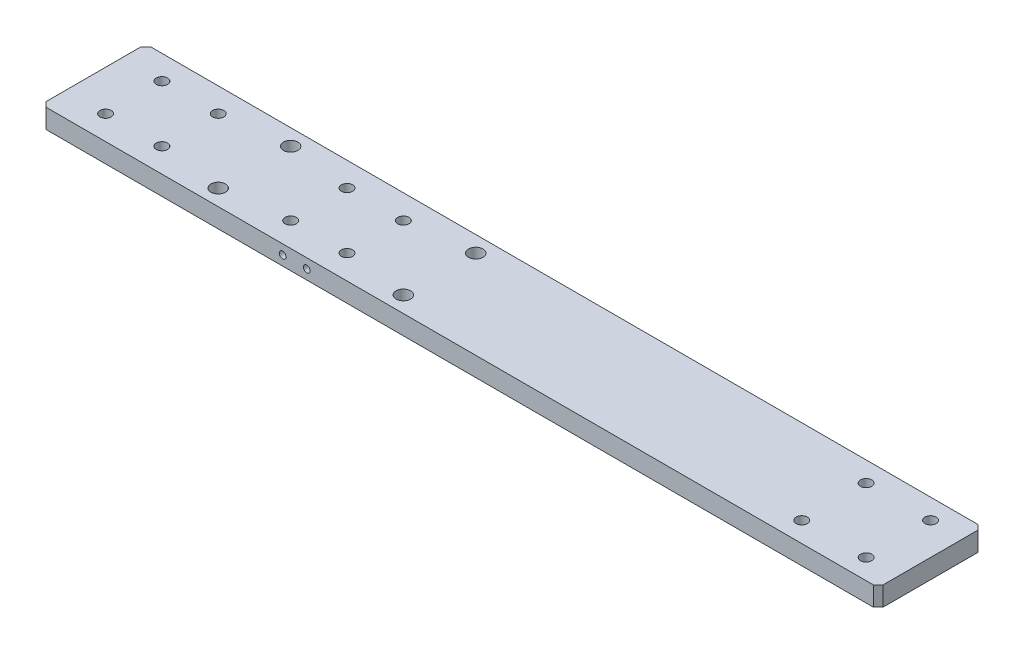
SolidWorks part; units mm, degrees
ref_plane "前视基准面" through (0, 0, 0) normal (0, 0, 1) x (1, 0, 0)
ref_plane "上视基准面" through (0, 0, 0) normal (0, 1, 0) x (1, 0, 0)
ref_plane "右视基准面" through (0, 0, 0) normal (1, 0, 0) x (0, 0, -1)
sketch "草图2" plane through (0, 0, 0) normal (0, 1, 0) x (1, 0, 0)
  line L1 (-260, 32.5) -> (260, 32.5)
  line L2 (-260, 32.5) -> (-260, -32.5)
  line L3 (-260, -32.5) -> (260, -32.5)
  line L4 (260, 32.5) -> (260, -32.5)
  line L5 (-260, 32.5) -> (260, -32.5) construction
  line L6 (-260, -32.5) -> (260, 32.5) construction
  point P0 (0, 0)
  dimension "D1" = 65
  dimension "D2" = 520
extrude "凸台-拉伸1" add sketch "草图2" along normal blind 12
hole_wizard "Ø7.0 (7) 直径孔1" positions "草图9" profile "草图8" hole size "Ø7.0" standard "GB" end condition through all
sketch "草图9" plane through (0, 0, 0) normal (0, 1, 0) x (1, 0, 0)
  line L0 (260, -32.5) -> (260, 32.5) construction
  point P0 (240, 20)
  point P2 (200, 20)
  point P4 (200, -20)
  point P6 (240, -20)
  dimension "D1" = 20
  dimension "D2" = 40
  dimension "D3" = 20
  dimension "D4" = 40
sketch "草图8" plane through (240, 0, -20) normal (1, 0, 0) x (0, 0, -1)
  line L0 (0, 0) -> (0, 12)
  line L1 (0, 12) -> (3.5, 12)
  line L2 (3.5, 12) -> (3.5, 0)
  line L5 (3.5, 0) -> (0, 0)
  line L11 (0, -6.35) -> (0, 107.95) construction
  dimension "通孔孔直径" = 7
  dimension "通孔孔深度" = 12
hole_wizard "M6 螺纹孔1" positions "草图11" profile "草图10" tap size "M6" standard "ISO"
sketch "草图11" plane through (-225, 0, 0) normal (-1, 0, 0) x (0, 0, 1)
  point P0 (0, 22)
  dimension "D1" = 22
cosmetic thread "孔螺蚊线1" [suppressed] parameters "D1"=17, "D2"=6
sketch "草图10" plane through (-225, 22, 0) normal (0, 1, 0) x (0, 0, 1)
  line L0 (0, 0) -> (0, 18.5022)
  line L1 (0, 18.5022) -> (2.5, 17)
  line L2 (2.5, 17) -> (2.5, 0)
  line L5 (2.5, 0) -> (0, 0)
  line L10 (0, 18.5022) -> (-2.5, 17) construction
  line L11 (0, -6.35) -> (0, 107.95) construction
  dimension "螺纹孔钻头直径" = 5
  dimension "螺纹孔钻头深度" = 17
  dimension "导头角度" = 118
chamfer "倒角1" distance 3 angle 45 4 edges at (260, 6, 32.5) (260, 6, -32.5) (-260, 6, 32.5) (-260, 6, -32.5)
hole_wizard "Ø9.0 (9) 直径孔2" positions "草图13" profile "草图12" hole size "Ø9.0" standard "GB" end condition through all
sketch "草图13" plane through (0, 12, 0) normal (0, 1, 0) x (1, 0, 0)
  point P0 (-160, -22.5)
  point P3 (-160, 22.5)
sketch "草图12" plane through (-160, 12, 22.5) normal (1, 0, 0) x (0, 0, 1)
  line L0 (0, 0) -> (0, 12)
  line L1 (0, 12) -> (4.5, 12)
  line L2 (4.5, 12) -> (4.5, 0)
  line L5 (4.5, 0) -> (0, 0)
  line L11 (0, -6.35) -> (0, 107.95) construction
  dimension "通孔孔直径" = 9
  dimension "通孔孔深度" = 12
hole_wizard "Ø9.0 (9) 直径孔1" positions "草图15" profile "草图14" hole size "Ø9.0" standard "GB" end condition through all
sketch "草图15" plane through (0, 12, 0) normal (0, 1, 0) x (1, 0, 0)
  line L0 (-260, 0) -> (-83.929, 0) construction
  line L1 (-260, 29.5) -> (-260, -29.5) construction
  point P0 (-235, -17.5)
  point P2 (-235, 17.5)
  point P4 (-200, -17.5)
  point P6 (-200, 17.5)
  dimension "D1" = 35
  dimension "D2" = 35
  dimension "D3" = 35
  dimension "D4" = 25
sketch "草图14" plane through (-235, 12, 17.5) normal (1, 0, 0) x (0, 0, 1)
  line L0 (0, 0) -> (0, 12)
  line L1 (0, 12) -> (3.5, 12)
  line L2 (3.5, 12) -> (3.5, 0)
  line L5 (3.5, 0) -> (0, 0)
  line L11 (0, -6.35) -> (0, 107.95) construction
  dimension "通孔孔直径" = 7
  dimension "通孔孔深度" = 12
pattern_linear "阵列(线性)1" count 2 spacing 115 along (1, 0, 0) of "Ø9.0 (9) 直径孔1"
hole_wizard "Ø9.0 (9) 直径孔3" positions "草图17" profile "草图16" hole size "Ø9.0" standard "GB" end condition through all
sketch "草图17" plane through (0, 12, 0) normal (0, 1, 0) x (1, 0, 0)
  point P0 (-45, -22.5)
  point P3 (-45, 22.5)
sketch "草图16" plane through (-45, 12, 22.5) normal (1, 0, 0) x (0, 0, 1)
  line L0 (0, 0) -> (0, 12)
  line L1 (0, 12) -> (4.5, 12)
  line L2 (4.5, 12) -> (4.5, 0)
  line L5 (4.5, 0) -> (0, 0)
  line L11 (0, -6.35) -> (0, 107.95) construction
  dimension "通孔孔直径" = 9
  dimension "通孔孔深度" = 12
hole_wizard "M5 螺纹孔1" positions "草图19" profile "草图20" tap size "M5" standard "ISO"
sketch "草图19" plane through (0, 0, -32.5) normal (0, 0, -1) x (-1, 0, 0)
  point P0 (95, 6)
  point P3 (110, 6)
sketch "草图20" plane through (-95, 6, -32.5) normal (1, 0, 0) x (0, 1, 0)
  line L0 (0, 0) -> (0, 13.6618)
  line L1 (0, 13.6618) -> (2.1, 12.4)
  line L2 (2.1, 12.4) -> (2.1, 0)
  line L5 (2.1, 0) -> (0, 0)
  line L10 (0, 13.6618) -> (-2.1, 12.4) construction
  line L11 (0, -6.35) -> (0, 107.95) construction
  dimension "螺纹孔钻头直径" = 4.2
  dimension "螺纹孔钻头深度" = 12.4
  dimension "导头角度" = 118
cosmetic thread "孔螺蚊线2" parameters "D1"=10, "D2"=5
cosmetic thread "孔螺蚊线3" parameters "D1"=10, "D2"=5
hole_wizard "M5 螺纹孔2" positions "草图22" profile "草图21" tap size "M5" standard "ISO"
sketch "草图22" plane through (0, 0, 32.5) normal (0, 0, 1) x (1, 0, 0)
  point P0 (-95, 6)
  point P3 (-110, 6)
sketch "草图21" plane through (-95, 6, 32.5) normal (1, 0, 0) x (0, -1, 0)
  line L0 (0, 0) -> (0, 13.6618)
  line L1 (0, 13.6618) -> (2.1, 12.4)
  line L2 (2.1, 12.4) -> (2.1, 0)
  line L5 (2.1, 0) -> (0, 0)
  line L10 (0, 13.6618) -> (-2.1, 12.4) construction
  line L11 (0, -6.35) -> (0, 107.95) construction
  dimension "螺纹孔钻头直径" = 4.2
  dimension "螺纹孔钻头深度" = 12.4
  dimension "导头角度" = 118
cosmetic thread "孔螺蚊线4" parameters "D1"=10, "D2"=5
cosmetic thread "孔螺蚊线5" parameters "D1"=10, "D2"=5
